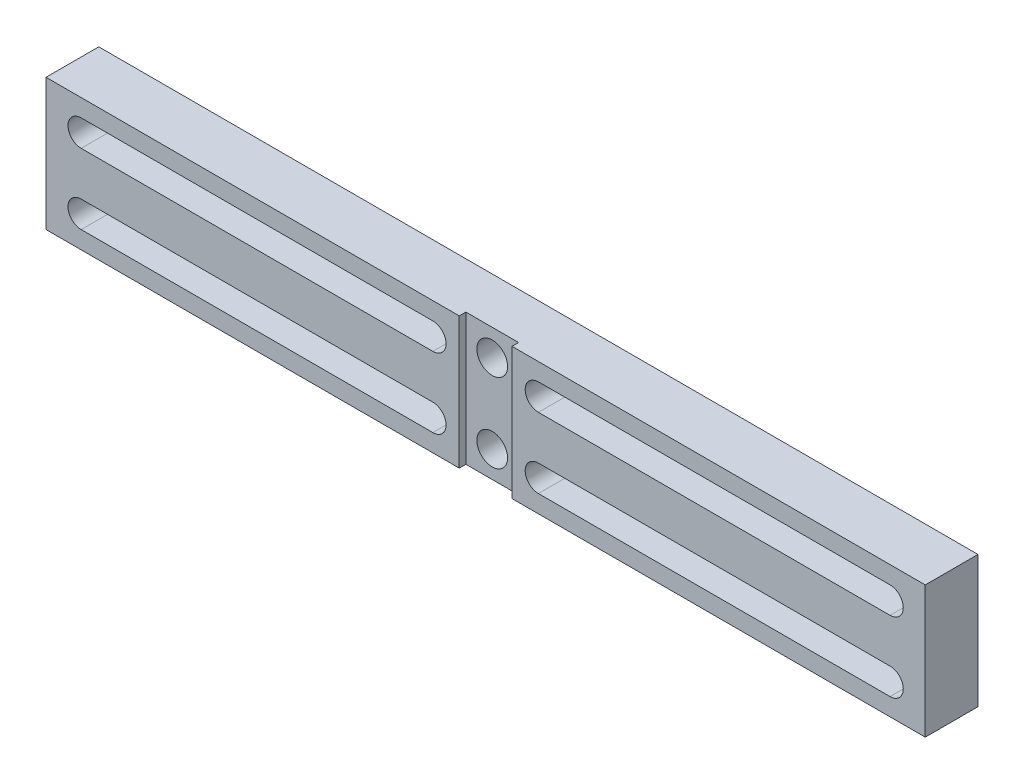
SolidWorks part; units mm, degrees
ref_plane "前视基准面" through (0, 0, 0) normal (0, 0, 1) x (1, 0, 0)
ref_plane "上视基准面" through (0, 0, 0) normal (0, 1, 0) x (1, 0, 0)
ref_plane "右视基准面" through (0, 0, 0) normal (1, 0, 0) x (0, 0, -1)
sketch "草图1" plane through (0, 0, 0) normal (0, 0, 1) x (1, 0, 0)
  line L0 (-92, 8) -> (-12, 8) construction
  line L1 (-100, -15) -> (100, -15)
  line L2 (-100, -15) -> (-100, 15)
  line L3 (-100, 15) -> (100, 15)
  line L4 (100, -15) -> (100, 15)
  line L5 (-100, -15) -> (100, 15) construction
  line L6 (-100, 15) -> (100, -15) construction
  line L7 (-92, 11) -> (-12, 11)
  line L8 (-92, 5) -> (-12, 5)
  line L9 (0, 0) -> (-100, 0) construction
  line L10 (-92, -8) -> (-12, -8) construction
  line L11 (-92, -11) -> (-12, -11)
  line L12 (-92, -5) -> (-12, -5)
  line L13 (0, 0) -> (0, -15) construction
  line L14 (92, 8) -> (12, 8) construction
  line L15 (92, 11) -> (12, 11)
  line L16 (92, 5) -> (12, 5)
  line L17 (92, -8) -> (12, -8) construction
  line L18 (92, -11) -> (12, -11)
  line L19 (92, -5) -> (12, -5)
  arc A0 (-92, 11) -> (-92, 5) centre (-92, 8) ccw
  arc A1 (-12, 5) -> (-12, 11) centre (-12, 8) ccw
  arc A2 (-92, -11) -> (-92, -5) centre (-92, -8) cw
  arc A3 (-12, -5) -> (-12, -11) centre (-12, -8) cw
  arc A4 (92, 11) -> (92, 5) centre (92, 8) cw
  arc A5 (12, 5) -> (12, 11) centre (12, 8) cw
  arc A6 (92, -11) -> (92, -5) centre (92, -8) ccw
  arc A7 (12, -5) -> (12, -11) centre (12, -8) ccw
  point P0 (0, 0)
  point P8 (-52, 8)
  point P17 (-52, -8)
  point P25 (52, 8)
  point P32 (52, -8)
  dimension "D3" = 3
  dimension "D1" = 30
  dimension "D2" = 200
  dimension "D4" = 4
  dimension "D5" = 8
  dimension "D6" = 12
extrude "凸台-拉伸1" add sketch "草图1" along normal blind 12
sketch "草图2" plane through (0, 0, 12) normal (0, 0, 1) x (1, 0, 0)
  line L0 (100, 15) -> (-100, 15) construction
  line L1 (-6, -15) -> (6, -15)
  line L2 (-6, -15) -> (-6, 15)
  line L3 (-6, 15) -> (6, 15)
  line L4 (6, -15) -> (6, 15)
  line L5 (-6, -15) -> (6, 15) construction
  line L6 (-6, 15) -> (6, -15) construction
  point P0 (0, 0)
  dimension "D1" = 12
extrude "切除-拉伸1" cut sketch "草图2" against normal blind 1.5
sketch "草图3" plane through (0, 0, 10.5) normal (0, 0, 1) x (1, 0, 0)
  line L0 (6, 15) -> (-6, 15) construction
  line L1 (-6, -15) -> (6, -15) construction
  circle A0 centre (0, 9) radius 3.5
  circle A1 centre (0, -9) radius 3.5
  dimension "D1" = 7
  dimension "D2" = 6
  dimension "D3" = 6
extrude "切除-拉伸2" cut sketch "草图3" against normal up to next
